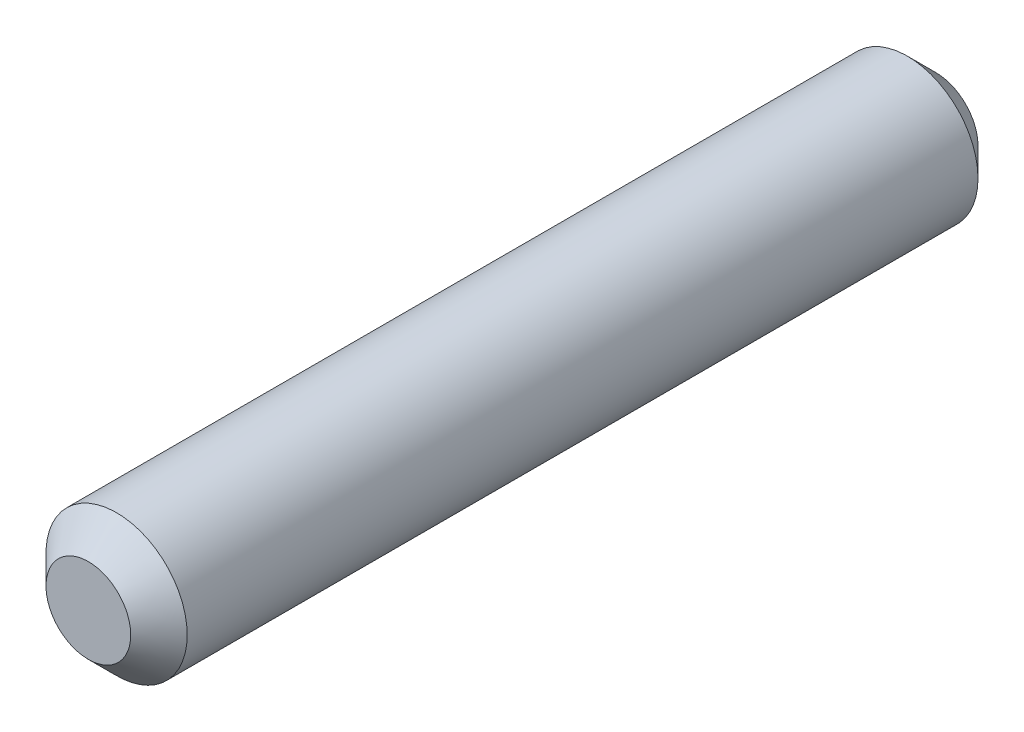
SolidWorks part; units mm, degrees
ref_plane "Front Plane" through (0, 0, 0) normal (0, 0, 1) x (1, 0, 0)
ref_plane "Top Plane" through (0, 0, 0) normal (0, 1, 0) x (1, 0, 0)
ref_plane "Right Plane" through (0, 0, 0) normal (1, 0, 0) x (0, 0, -1)
sketch "Sketch1" plane through (0, 0, 0) normal (0, 0, 1) x (1, 0, 0)
  circle A0 centre (0, 0) radius 2.5
  dimension "D1" = 5
extrude "Boss-Extrude1" add sketch "Sketch1" along normal blind 30
chamfer "Chamfer1" distance 1 angle 45 2 edges at (2.5, 0, 0) (2.5, 0, 30)
